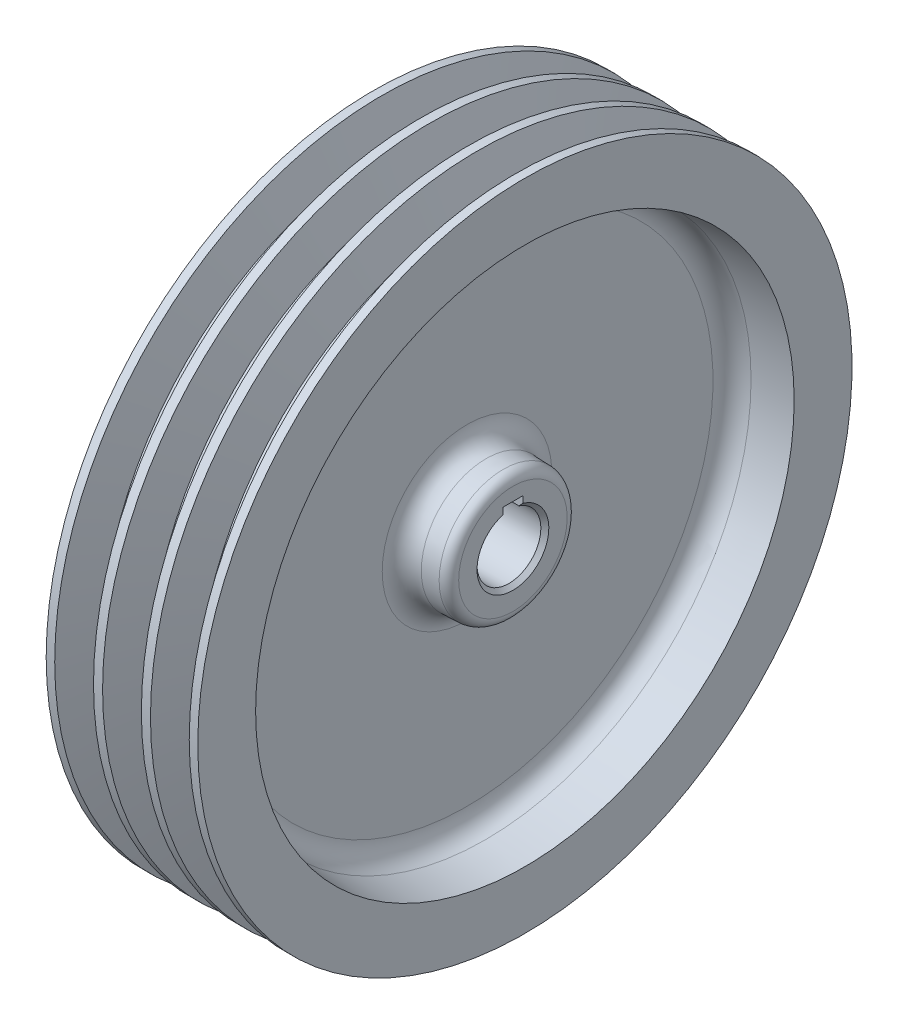
SolidWorks part; units mm, degrees
ref_plane "前视基准面" through (0, 0, 0) normal (0, 0, 1) x (1, 0, 0)
ref_plane "上视基准面" through (0, 0, 0) normal (0, 1, 0) x (1, 0, 0)
ref_plane "右视基准面" through (0, 0, 0) normal (1, 0, 0) x (0, 0, -1)
sketch "草图1" plane through (0, 0, 0) normal (0, 0, 1) x (1, 0, 0)
  line L0 (0, 0) -> (64.8368, 0) construction
  line L1 (3, 8) -> (3, 16)
  line L2 (0, 82) -> (38, 82)
  line L3 (38, 82) -> (38, 67.5)
  line L4 (3, 16) -> (-44, 16) construction
  line L5 (14.5, 17.0061) -> (14.5, 66.9202)
  line L6 (35, 8) -> (3, 8)
  line L7 (2.1385, 82) -> (4.8901, 73) construction
  line L8 (4.8901, 73) -> (9.1099, 73) construction
  line L9 (9.1099, 73) -> (11.8615, 82) construction
  line L10 (0, 80) -> (38, 80) construction
  line L11 (7, 73) -> (7, 8) construction
  line L12 (44, 67.5) -> (0, 67.5) construction
  line L13 (38, 67.5) -> (79, 67.5) construction
  line L14 (23.5, 66.2314) -> (23.5, 16.4599)
  line L15 (-9, 16) -> (35, 16) construction
  line L16 (19, 8) -> (19, 82) construction
  line L17 (35, 16) -> (35, 8)
  line L18 (0, 67.5) -> (0, 82)
  line L19 (14.5, 54.5) -> (23.5, 54.5) construction
  line L20 (14.5, 29) -> (23.5, 29) construction
  line L21 (38, 67.5) -> (38, 54.5) construction
  line L22 (38, 54.5) -> (23.5, 54.5) construction
  line L23 (23.5, 29) -> (35, 29) construction
  line L24 (35, 29) -> (35, 16) construction
  line L25 (23.5, 66.2314) -> (38, 67.5)
  line L26 (14.5, 66.9202) -> (0, 67.5)
  line L27 (14.5, 17.0061) -> (3, 16)
  line L28 (23.5, 16.4599) -> (35, 16)
  point P17 (2.75, 80)
  point P18 (11.25, 80)
  dimension "d2" = 135
  dimension "L" = 32
  dimension "B" = 38
  dimension "d" = 16
  dimension "d1" = 32
  dimension "D3" = 5
  dimension "D4" = 2.29
  dimension "dd" = 160
  dimension "f" = 7
  dimension "槽轮角" = 34
  dimension "bd" = 8.5
  dimension "hf" = 7
  dimension "ha" = 2
  dimension "da" = 164
  dimension "S" = 9
  dimension "S2" = 13
revolve "旋转1" add sketch "草图1" angle 360 about L0
sketch "草图2" plane through (0, 0, 0) normal (0, 0, 1) x (1, 0, 0)
  line L0 (9.1099, 73) -> (11.8615, 82) construction
  line L1 (4.8901, 73) -> (9.1099, 73) construction
  line L2 (2.1385, 82) -> (4.8901, 73) construction
  line L3 (9.1099, 73) -> (11.8615, 82)
  line L4 (4.8901, 73) -> (9.1099, 73)
  line L5 (2.1385, 82) -> (4.8901, 73)
  line L6 (2.1385, 82) -> (11.8615, 82)
  line L7 (0, 0) -> (123, 0) construction
revolve "切除-旋转1" cut sketch "草图2" angle 360 about L7
pattern_linear "轮槽数" count 3 spacing 12 along (1, 0, 0) of "切除-旋转1"
chamfer "倒角1" distance 1 2 edges at (3, 0, 8) (35, 0, 8)
sketch "草图4" plane through (3, 0, 0) normal (-1, 0, 0) x (0, 0, 1)
  line L1 (-2.5, 7.5993) -> (2.5, 7.5993)
  line L2 (-2.5, 7.5993) -> (-2.5, 10.3)
  line L3 (-2.5, 10.3) -> (2.5, 10.3)
  line L4 (2.5, 7.5993) -> (2.5, 10.3)
  circle A0 centre (0, 0) radius 8 construction
  point P6 (0.2, 10.3)
  dimension "键槽高度" = 10.3
  dimension "键槽宽度" = 5
  dimension "t1" = 2.3
extrude "切除-拉伸1" cut sketch "草图4" against normal through all
fillet "圆角1" radius 5 4 edges at (23.5, 0, 66.2314) (14.5, 0, 17.0061) (14.5, 0, 66.9202) (23.5, 0, 16.4599)
fillet "圆角2" radius 2.5 2 edges at (35, 0, 16) (3, 0, 16)
